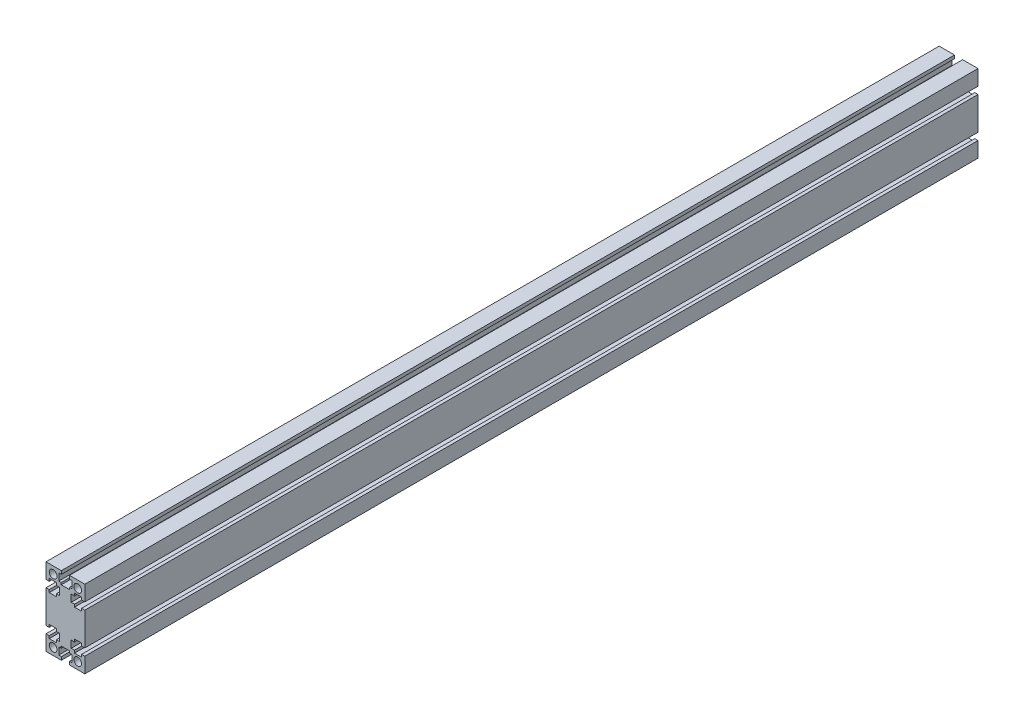
SolidWorks part; units mm, degrees
ref_plane "前视基准面" through (0, 0, 0) normal (0, 0, 1) x (1, 0, 0)
ref_plane "上视基准面" through (0, 0, 0) normal (0, 1, 0) x (1, 0, 0)
ref_plane "右视基准面" through (0, 0, 0) normal (1, 0, 0) x (0, 0, -1)
sketch "草图1" plane through (0, 0, 0) normal (0, 0, 1) x (1, 0, 0)
  line L0 (-27.4957, 11.1925) -> (-24.9957, 11.1925)
  line L1 (-27.4957, 23.0425) -> (-15.6457, 23.0425)
  line L2 (-27.4957, 23.0425) -> (-27.4957, 11.1925)
  line L3 (-27.4957, -36.9575) -> (-15.6457, -36.9575)
  line L4 (2.5043, 23.0425) -> (2.5043, 11.1925)
  line L5 (-24.9957, 11.1925) -> (-24.9957, 13.1925)
  line L6 (-24.9957, 13.1925) -> (-19.4957, 13.1925)
  line L7 (-19.4957, 13.1925) -> (-19.4957, 11.1925)
  line L14 (-24.9957, 5.6925) -> (-27.4957, 5.6925)
  line L15 (-27.4957, 5.6925) -> (-27.4957, -19.6075)
  line L18 (-19.4957, 5.6925) -> (-16.9957, 5.6925)
  line L19 (-16.9957, 5.6925) -> (-16.9957, 11.1925)
  line L20 (-16.9957, 11.1925) -> (-19.4957, 11.1925)
  line L21 (-24.9957, 5.6925) -> (-24.9957, 3.6925)
  line L22 (-24.9957, 3.6925) -> (-19.4957, 3.6925)
  line L23 (-19.4957, 3.6925) -> (-19.4957, 5.6925)
  line L24 (-12.4957, 23.0425) -> (-12.4957, 50023.0425) construction
  line L25 (0.0043, 5.6925) -> (2.5043, 5.6925)
  line L26 (0.0043, 5.6925) -> (0.0043, 3.6925)
  line L27 (0.0043, 3.6925) -> (-5.4957, 3.6925)
  line L28 (-5.4957, 3.6925) -> (-5.4957, 5.6925)
  line L29 (-5.4957, 5.6925) -> (-7.9957, 5.6925)
  line L30 (-7.9957, 5.6925) -> (-7.9957, 11.1925)
  line L31 (-7.9957, 11.1925) -> (-5.4957, 11.1925)
  line L32 (-5.4957, 13.1925) -> (-5.4957, 11.1925)
  line L33 (2.5043, 11.1925) -> (0.0043, 11.1925)
  line L34 (0.0043, 11.1925) -> (0.0043, 13.1925)
  line L35 (0.0043, 13.1925) -> (-5.4957, 13.1925)
  line L36 (2.5043, 5.6925) -> (2.5043, -19.6075)
  line L37 (-15.6457, 23.0425) -> (-15.6457, 20.5425)
  line L38 (-15.6457, 20.5425) -> (-17.6457, 20.5425)
  line L39 (-17.6457, 20.5425) -> (-17.6457, 15.0425)
  line L40 (-17.6457, 15.0425) -> (-15.7481, 15.0425)
  line L41 (-15.7481, 15.0425) -> (-15.7481, 13.5076)
  line L42 (-15.7481, 13.5076) -> (-9.2434, 13.5076)
  line L43 (-9.3457, 23.0425) -> (2.5043, 23.0425)
  line L45 (-9.2434, 15.0425) -> (-9.2434, 13.5076)
  line L46 (-7.3457, 15.0425) -> (-9.2434, 15.0425)
  line L47 (-9.3457, 20.5425) -> (-7.3457, 20.5425)
  line L48 (-7.3457, 20.5425) -> (-7.3457, 15.0425)
  line L49 (-9.3457, 23.0425) -> (-9.3457, 20.5425)
  line L50 (-9.3457, -36.9575) -> (-9.3457, -34.4575)
  line L51 (-9.3457, -34.4575) -> (-7.3457, -34.4575)
  line L52 (48.9171, -6.9575) -> (-49951.0829, -6.9575) construction
  line L53 (-7.3457, -34.4575) -> (-7.3457, -28.9575)
  line L54 (-7.3457, -28.9575) -> (-9.2434, -28.9575)
  line L55 (-9.2434, -28.9575) -> (-9.2434, -27.4226)
  line L56 (-5.4957, -27.1075) -> (-5.4957, -25.1075)
  line L57 (0.0043, -27.1075) -> (-5.4957, -27.1075)
  line L58 (0.0043, -25.1075) -> (0.0043, -27.1075)
  line L59 (2.5043, -25.1075) -> (0.0043, -25.1075)
  line L60 (0.0043, -19.6075) -> (2.5043, -19.6075)
  line L61 (0.0043, -19.6075) -> (0.0043, -17.6075)
  line L62 (-5.4957, -17.6075) -> (-5.4957, -19.6075)
  line L63 (0.0043, -17.6075) -> (-5.4957, -17.6075)
  line L64 (-5.4957, -19.6075) -> (-7.9957, -19.6075)
  line L65 (-7.9957, -19.6075) -> (-7.9957, -25.1075)
  line L66 (-7.9957, -25.1075) -> (-5.4957, -25.1075)
  line L67 (-15.7481, -27.4226) -> (-9.2434, -27.4226)
  line L68 (-15.7481, -28.9575) -> (-15.7481, -27.4226)
  line L69 (-17.6457, -28.9575) -> (-15.7481, -28.9575)
  line L70 (-15.6457, -36.9575) -> (-15.6457, -34.4575)
  line L71 (-15.6457, -34.4575) -> (-17.6457, -34.4575)
  line L72 (-17.6457, -34.4575) -> (-17.6457, -28.9575)
  line L73 (-24.9957, -27.1075) -> (-19.4957, -27.1075)
  line L74 (-19.4957, -27.1075) -> (-19.4957, -25.1075)
  line L75 (-16.9957, -25.1075) -> (-19.4957, -25.1075)
  line L76 (-16.9957, -19.6075) -> (-16.9957, -25.1075)
  line L77 (-19.4957, -19.6075) -> (-16.9957, -19.6075)
  line L78 (-19.4957, -17.6075) -> (-19.4957, -19.6075)
  line L79 (-24.9957, -17.6075) -> (-19.4957, -17.6075)
  line L80 (-24.9957, -19.6075) -> (-24.9957, -17.6075)
  line L81 (-24.9957, -25.1075) -> (-24.9957, -27.1075)
  line L82 (-27.4957, -25.1075) -> (-24.9957, -25.1075)
  line L83 (-24.9957, -19.6075) -> (-27.4957, -19.6075)
  line L84 (-27.4957, -25.1075) -> (-27.4957, -36.9575)
  line L85 (2.5043, -25.1075) -> (2.5043, -36.9575)
  line L86 (-9.3457, -36.9575) -> (2.5043, -36.9575)
  circle A0 centre (-21.9957, 17.5425) radius 3
  circle A1 centre (-2.9957, 17.5425) radius 3
  circle A2 centre (-2.9957, -31.4575) radius 3
  circle A3 centre (-21.9957, -31.4575) radius 3
  point P43 (-12.4957, 13.5076)
  dimension "D14" = 6
  dimension "D1" = 60
  dimension "D2" = 30
  dimension "D3" = 11.85
  dimension "D4" = 2.5
  dimension "D5" = 2
  dimension "D6" = 5.5
  dimension "D7" = 2
  dimension "D8" = 2.5
  dimension "D9" = 5.5
  dimension "D10" = 2.5
  dimension "D11" = 2
  dimension "D12" = 2
  dimension "D13" = 5.5
  dimension "D15" = 5.5
  dimension "D16" = 5.5
  dimension "D17" = 6.3
  dimension "D18" = 2.5
  dimension "D19" = 2
  dimension "D20" = 5.5
  dimension "D21" = 1.8977
extrude "凸台-拉伸1" add sketch "草图1" along normal blind 690
